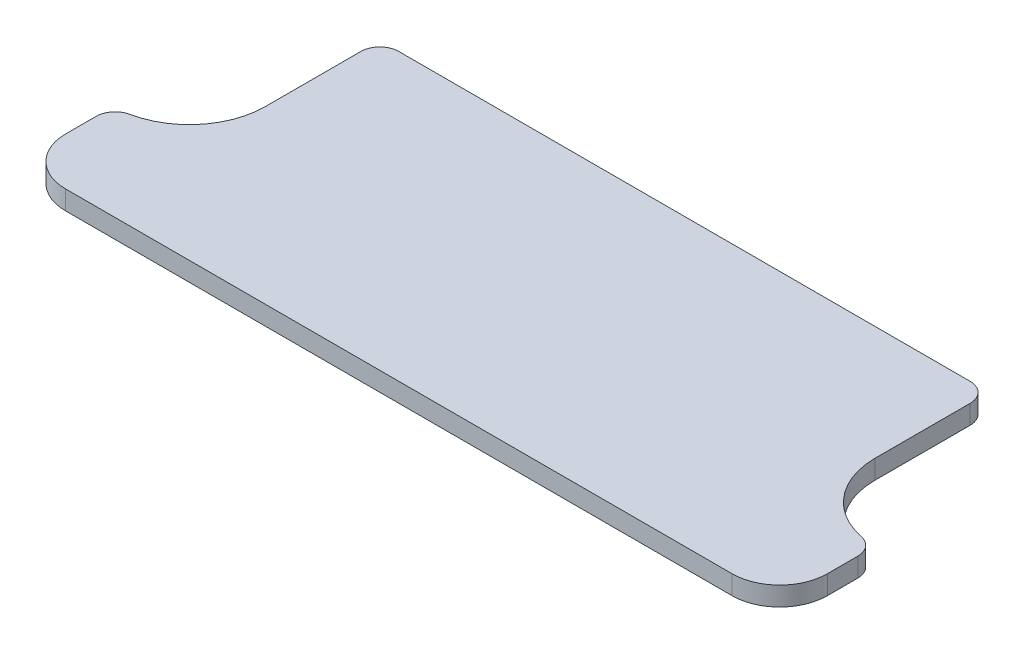
SolidWorks part; units mm, degrees
ref_plane "Front Plane" through (0, 0, 0) normal (0, 0, 1) x (1, 0, 0)
ref_plane "Top Plane" through (0, 0, 0) normal (0, 1, 0) x (1, 0, 0)
ref_plane "Right Plane" through (0, 0, 0) normal (1, 0, 0) x (0, 0, -1)
other "Configuration Table"
sketch "Sketch1" plane through (0, 0, 0) normal (0, 1, 0) x (1, 0, 0)
  line L0 (-320, 150) -> (-320, 30)
  line L1 (-320, 150) -> (320, 150)
  line L2 (-400, -50) -> (-400, -150)
  line L3 (-400, -150) -> (400, -150)
  line L4 (400, -50) -> (400, -150)
  line L5 (-400, 150) -> (400, -150) construction
  line L6 (-400, -150) -> (400, 150) construction
  line L7 (0, 0) -> (0, 276.8059) construction
  line L8 (320, 150) -> (320, 30)
  arc A0 (-320, 30) -> (-400, -50) centre (-400, 30) cw
  arc A1 (320, 30) -> (400, -50) centre (400, 30) ccw
  point P0 (0, 0)
  dimension "D1" = 800
  dimension "D2" = 300
  dimension "D3" = 300
  dimension "D4" = 150
  dimension "D5" = 80
  dimension "D6" = 200
  dimension "D7" = 150
extrude "Boss-Extrude1" add sketch "Sketch1" against normal blind 20
fillet "Fillet1" radius 50 2 edges at (400, -10, 150) (-400, -10, 150)
fillet "Fillet2" radius 20 4 edges at (400, -10, 50) (-400, -10, 50) (-320, -10, -150) (320, -10, -150)
